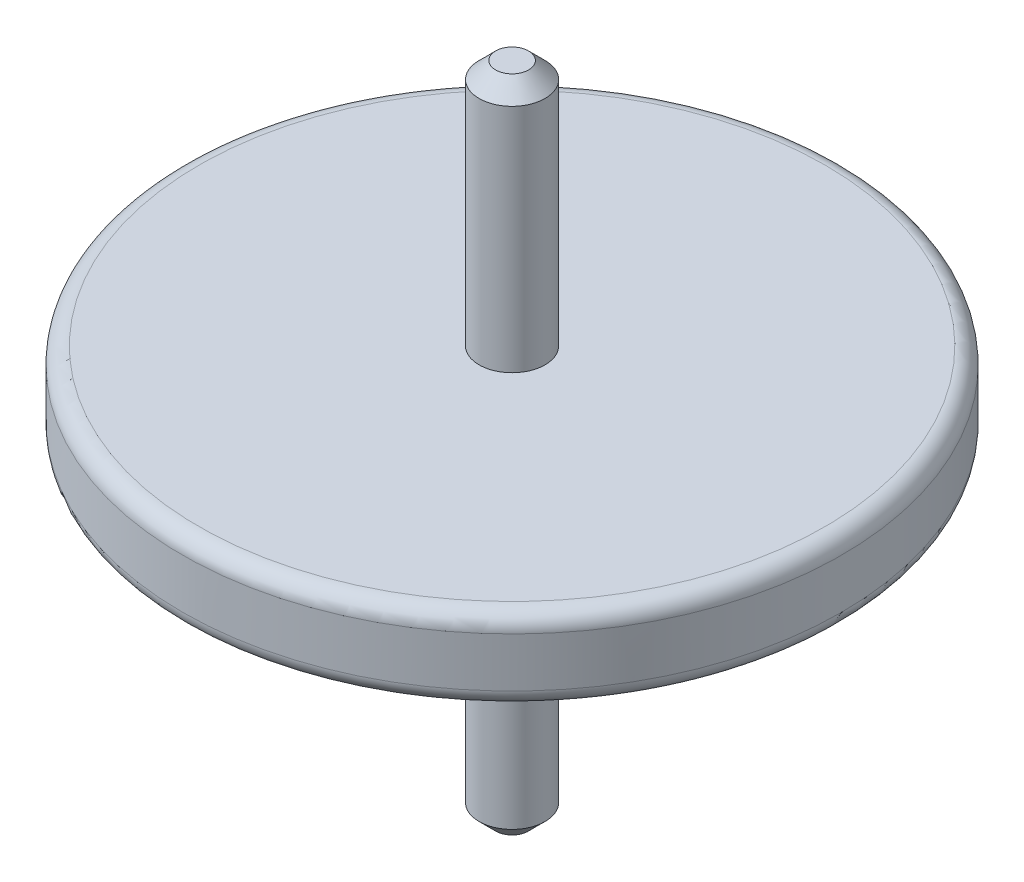
from build123d import *

# Parameters (mm, degrees)
CHAMFER1_SIZE = 1
FILLET1_R     = 1


with BuildPart() as part:
    # Sketch1 → Revolve1 (revolve)
    with BuildSketch(Plane.XY, mode=Mode.PRIVATE) as revolve1_sk:
        Polygon((0, 40), (-2, 40), (-2, 25), (-20, 25), (-20, 20), (-6, 20), (-6, 15), (-2, 15), (-2, 0), (0, 0), align=None)
    revolve(revolve1_sk.sketch.rotate(Axis((0, 0, 0), (0, 1, 0)), 270), axis=Axis((0, 0, 0), (0, 1, 0)))

    # Chamfer1
    chamfer1_edges = [part.edges().sort_by_distance(p)[0] for p in [
        (0, 40, 2),
        (0, 0, 2),
    ]]
    chamfer(chamfer1_edges, length=CHAMFER1_SIZE)

    # Fillet1
    fillet1_edges = [part.edges().sort_by_distance(p)[0] for p in [
        (0, 20, 20),
        (0, 25, 20),
    ]]
    fillet(fillet1_edges, radius=FILLET1_R)


solid = part.part
